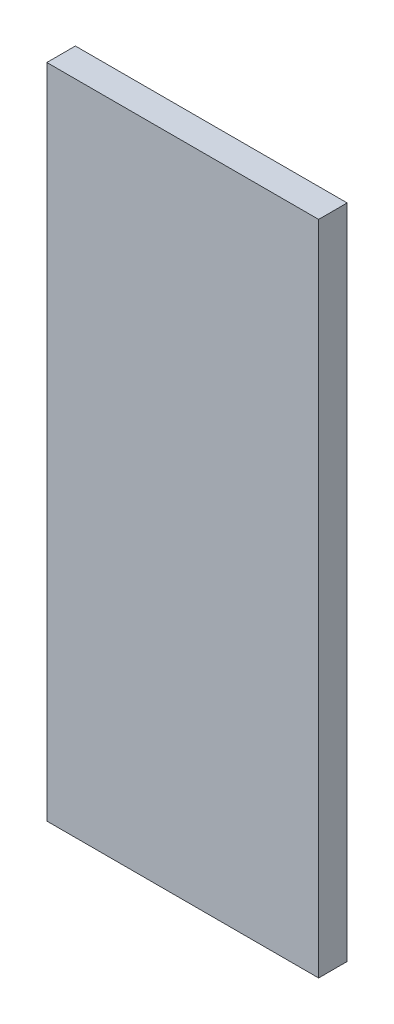
from build123d import *

# Parameters (mm, degrees)
SKETCH1_W           = 76.2
SKETCH1_H           = 184.2
BOSS_EXTRUDE1_DEPTH = 4


with BuildPart() as part:
    # Sketch1 → Boss-Extrude1 (new, symmetric)
    with BuildSketch(Plane.XY):
        Rectangle(SKETCH1_W, SKETCH1_H)
    extrude(amount=BOSS_EXTRUDE1_DEPTH, both=True)


solid = part.part
